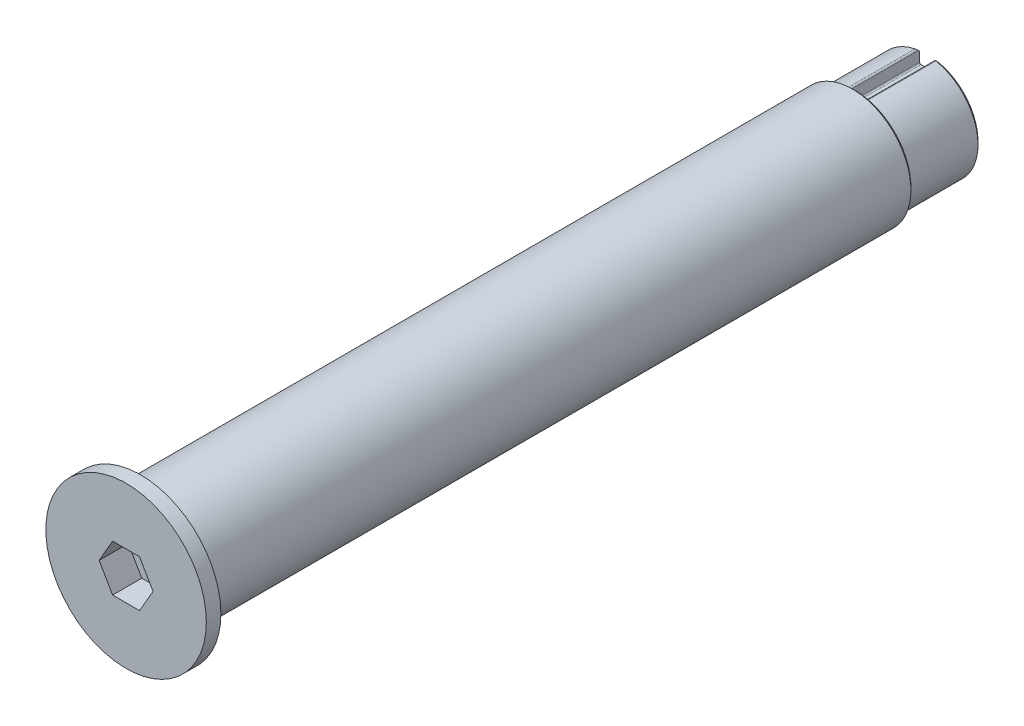
from build123d import *

# Parameters (mm, degrees)
SKETCH_1_R          = 20
EXTRUDE_1_DEPTH     = 270
SKETCH_2_R          = 27.5
EXTRUDE_2_DEPTH     = 5
CUT_EXTRUDE_1_DEPTH = 10
SKETCH_4_OUTSIDE_W  = 114.158
SKETCH_4_OUTSIDE_H  = 114.158
SKETCH_4_OUTSIDE_R  = 18
CUT_EXTRUDE_2_DEPTH = 25
CHAMFER_1_SIZE      = 1
CHAMFER_2_SIZE      = 1
FILLET_1_R          = 0.5
SKETCH_5_W          = 6
SKETCH_5_H          = 10
CUT_EXTRUDE_3_DEPTH = 25
FILLET_2_R          = 0.5


with BuildPart() as part:
    # 草图1 → 凸台-拉伸1 (new body)
    with BuildSketch(Plane.XY):
        Circle(SKETCH_1_R)
    extrude(amount=EXTRUDE_1_DEPTH)

    # 草图2 → 凸台-拉伸2 (add)
    with BuildSketch(Plane.XY.offset(270)):
        Circle(SKETCH_2_R)
    extrude(amount=EXTRUDE_2_DEPTH)

    # 草图3 → 切除-拉伸1 (cut)
    with BuildSketch(Plane.XY.offset(275)):
        Polygon((9.237604307, 0), (4.618802154, 8), (-4.618802154, 8), (-9.237604307, 0), (-4.618802154, -8), (4.618802154, -8), align=None)
    extrude(amount=-CUT_EXTRUDE_1_DEPTH, mode=Mode.SUBTRACT)

    # 草图4 outside → 切除-拉伸2 (cut)
    with BuildSketch(Plane(origin=(0, 0, 0), x_dir=(-1, 0, 0), z_dir=(0, 0, -1))):
        Rectangle(SKETCH_4_OUTSIDE_W, SKETCH_4_OUTSIDE_H)
        Circle(SKETCH_4_OUTSIDE_R, mode=Mode.SUBTRACT)
    extrude(amount=-CUT_EXTRUDE_2_DEPTH, mode=Mode.SUBTRACT)

    # 倒角1
    chamfer_1_edges = [part.edges().sort_by_distance(p)[0] for p in [
        (-20, 0, 25),
    ]]
    chamfer(chamfer_1_edges, length=CHAMFER_1_SIZE)

    # 倒角2
    chamfer_2_edges = [part.edges().sort_by_distance(p)[0] for p in [
        (18, 0, 0),
    ]]
    chamfer(chamfer_2_edges, length=CHAMFER_2_SIZE)

    # 圆角1
    fillet_1_edges = [part.edges().sort_by_distance(p)[0] for p in [
        (-20, 0, 270),
    ]]
    fillet(fillet_1_edges, radius=FILLET_1_R)

    # 草图5 → 切除-拉伸3 (cut)
    with BuildSketch(Plane(origin=(0, 0, 0), x_dir=(-1, 0, 0), z_dir=(0, 0, -1))):
        with Locations((0, 18)):
            Rectangle(SKETCH_5_W, SKETCH_5_H)
    extrude(amount=-CUT_EXTRUDE_3_DEPTH, mode=Mode.SUBTRACT)

    # 圆角2
    fillet_2_edges = [part.edges().sort_by_distance(p)[0] for p in [
        (3, 13, 12.5),
        (-3, 13, 12.5),
        (-3, 17.748239349, 13),
        (3, 17.748239349, 13),
    ]]
    fillet(fillet_2_edges, radius=FILLET_2_R)


solid = part.part
